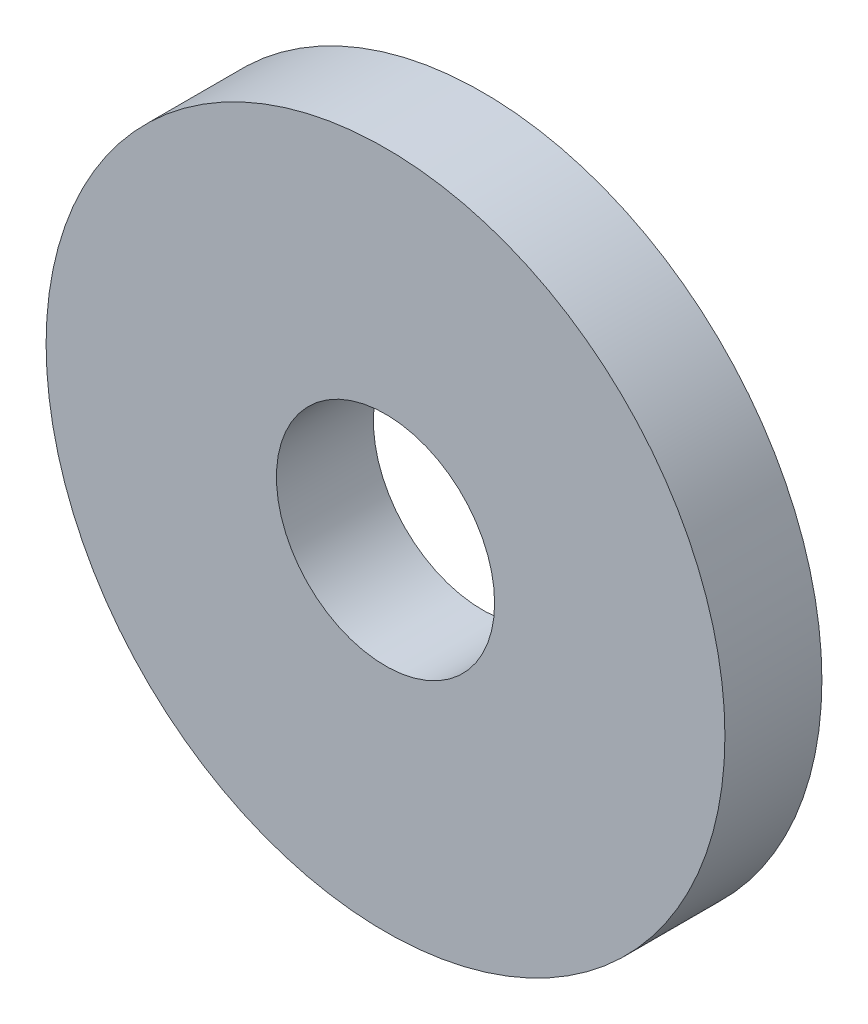
from build123d import *

# Parameters (mm, degrees)
SKETCH1_R           = 7
SKETCH1_R_2         = 2.25
BOSS_EXTRUDE1_DEPTH = 2


with BuildPart() as part:
    # Sketch1 → Boss-Extrude1 (new body)
    with BuildSketch(Plane.XY):
        Circle(SKETCH1_R)
        Circle(SKETCH1_R_2, mode=Mode.SUBTRACT)
    extrude(amount=BOSS_EXTRUDE1_DEPTH)


solid = part.part
